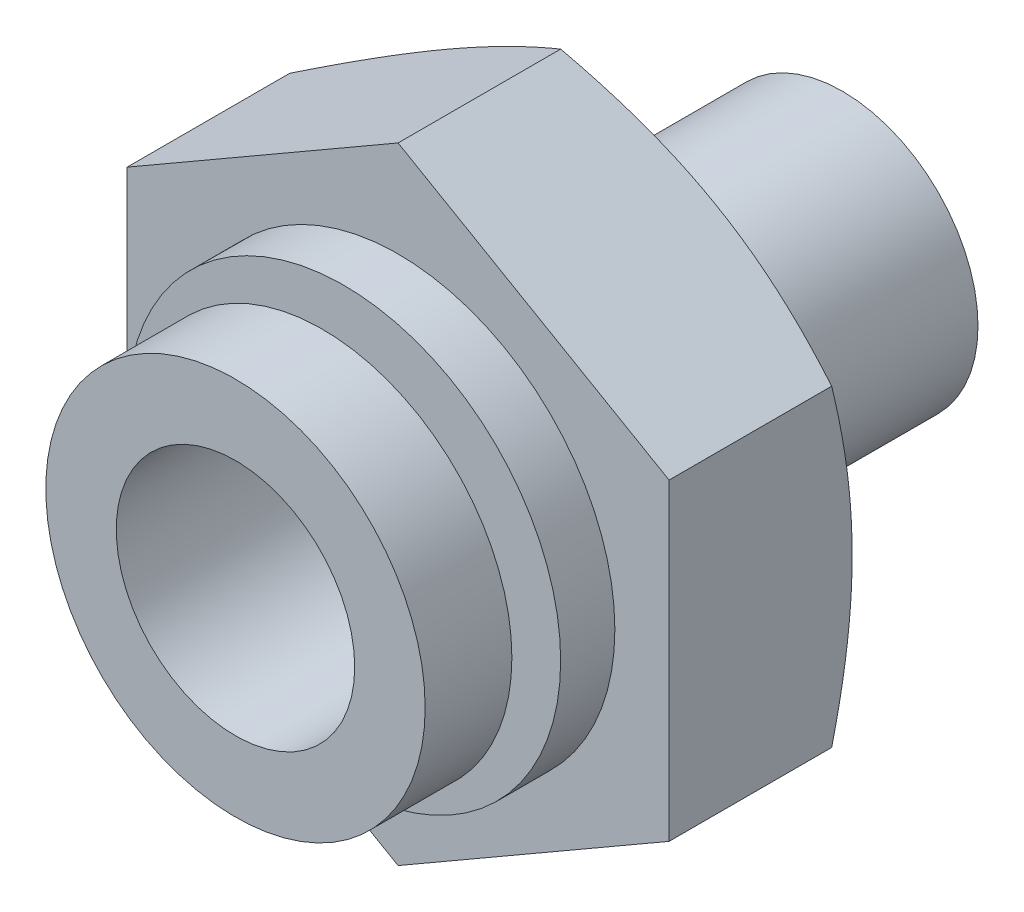
from build123d import *

# Parameters (mm, degrees)
BOSS_EXTRUDE1_DEPTH = 11.5
SKETCH4_R           = 12.5
BOSS_EXTRUDE2_DEPTH = 18
SKETCH5_R           = 20
BOSS_EXTRUDE3_DEPTH = 5
SKETCH6_R           = 14
BOSS_EXTRUDE4_DEPTH = 2
SKETCH7_R           = 17.5
BOSS_EXTRUDE5_DEPTH = 8
SKETCH8_R           = 11
CUT_EXTRUDE1_DEPTH  = 28
SKETCH9_R           = 10
CUT_EXTRUDE2_DEPTH  = 71


with BuildPart() as part:
    # Sketch1 → Boss-Extrude1 (new, symmetric)
    with BuildSketch(Plane.XY):
        Polygon((0, 28.867513459), (-25, 14.43375673), (-25, -14.43375673), (0, -28.867513459), (25, -14.43375673), (25, 14.43375673), align=None)
    extrude(amount=BOSS_EXTRUDE1_DEPTH, both=True)

    # Sketch3 → Cut-Revolve1 (revolve, cut)
    with BuildSketch(Plane(origin=(0, 0, 0), x_dir=(0, 0, -1), z_dir=(1, 0, 0)), mode=Mode.PRIVATE) as cut_revolve1_sk:
        Polygon((11.5, 12.5), (3.5, 28.867513459), (11.5, 28.867513459), align=None)
    revolve(cut_revolve1_sk.sketch.rotate(Axis((0, 0, 1000), (0, 0, -1)), 90), axis=Axis((0, 0, 1000), (0, 0, -1)), mode=Mode.SUBTRACT)

    # Sketch4 → Boss-Extrude2 (add)
    with BuildSketch(Plane(origin=(0, 0, -11.5), x_dir=(-1, 0, 0), z_dir=(0, 0, -1))):
        Circle(SKETCH4_R)
    extrude(amount=BOSS_EXTRUDE2_DEPTH)

    # Sketch5 → Boss-Extrude3 (add)
    with BuildSketch(Plane.XY.offset(11.5)):
        Circle(SKETCH5_R)
    extrude(amount=BOSS_EXTRUDE3_DEPTH)

    # Sketch6 → Boss-Extrude4 (add)
    with BuildSketch(Plane.XY.offset(16.5)):
        Circle(SKETCH6_R)
    extrude(amount=BOSS_EXTRUDE4_DEPTH)

    # Sketch7 → Boss-Extrude5 (add)
    with BuildSketch(Plane.XY.offset(18.5)):
        Circle(SKETCH7_R)
    extrude(amount=BOSS_EXTRUDE5_DEPTH)

    # Sketch8 → Cut-Extrude1 (cut)
    with BuildSketch(Plane.XY.offset(26.5)):
        Circle(SKETCH8_R)
    extrude(amount=-CUT_EXTRUDE1_DEPTH, mode=Mode.SUBTRACT)

    # Sketch9 → Cut-Extrude2 (cut)
    with BuildSketch(Plane(origin=(0, 0, -29.5), x_dir=(-1, 0, 0), z_dir=(0, 0, -1))):
        Circle(SKETCH9_R)
    extrude(amount=-CUT_EXTRUDE2_DEPTH, mode=Mode.SUBTRACT)


solid = part.part
